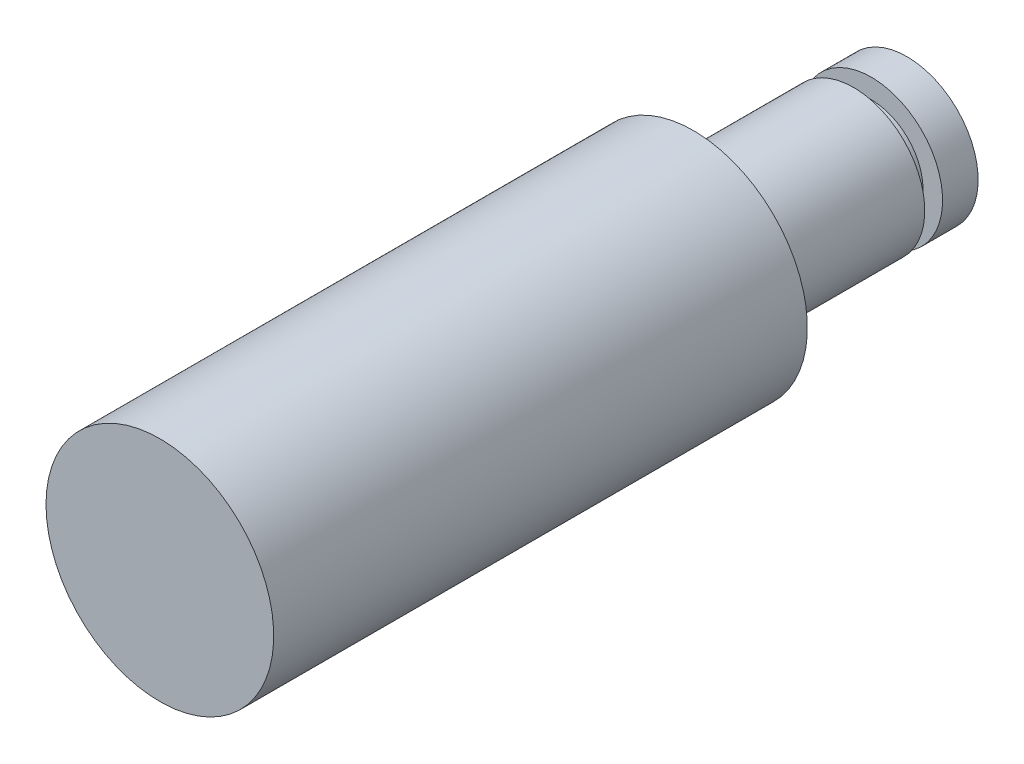
from build123d import *


with BuildPart() as part:
    # 草图1 → 旋转1 (revolve)
    with BuildSketch(Plane(origin=(0, 0, 0), x_dir=(1, 0, 0), z_dir=(0, 1, 0))):
        Polygon((0, 0), (-4, 0), (-4, -2), (-2.9, -2), (-2.9, -3), (-4, -3), (-4, -12), (-6.4, -12), (-6.4, -42), (0, -42), align=None)
    revolve(axis=Axis((0, 0, 0), (0, 0, 1)))


solid = part.part
